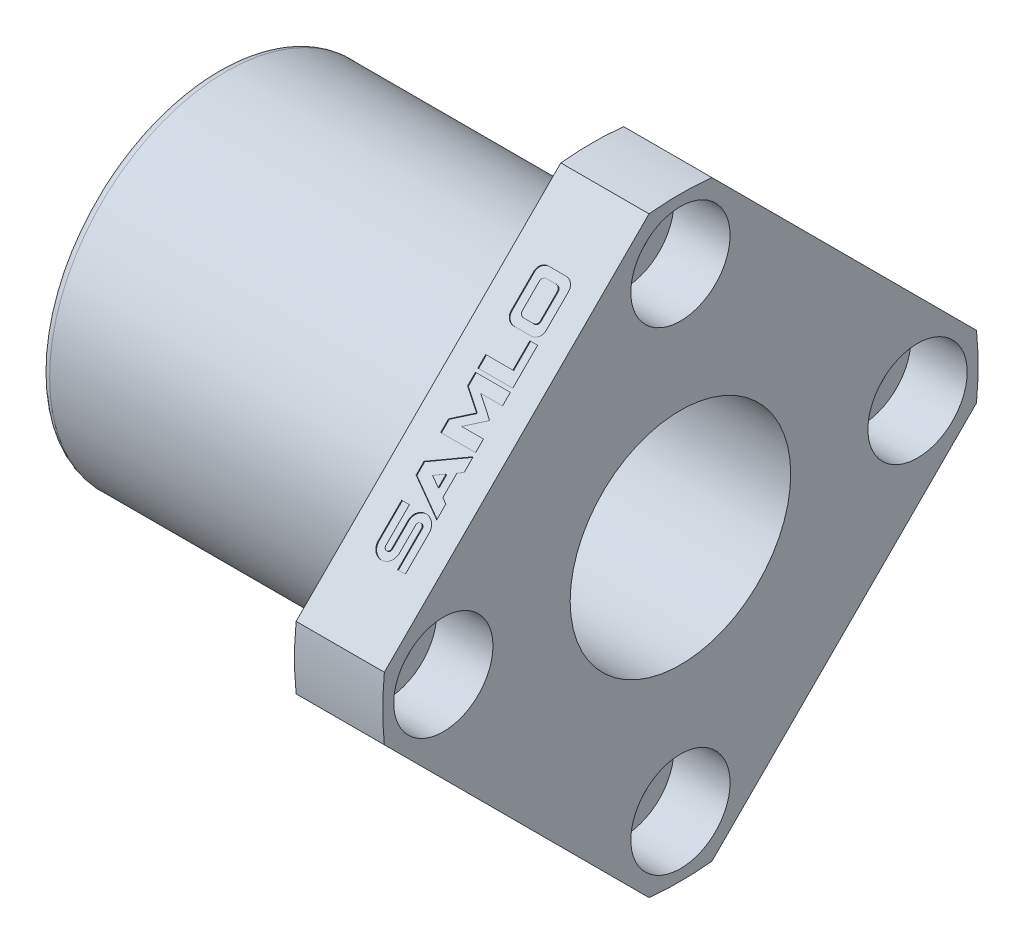
SolidWorks part; units mm, degrees
ref_plane "Front Plane" through (0, 0, 0) normal (0, 0, 1) x (1, 0, 0)
ref_plane "Top Plane" through (0, 0, 0) normal (0, 1, 0) x (1, 0, 0)
ref_plane "Right Plane" through (0, 0, 0) normal (1, 0, 0) x (0, 0, -1)
sketch "Sketch1" plane through (0, 0, 0) normal (0, 0, 1) x (1, 0, 0)
  line L0 (0, 10) -> (42, 10)
  line L1 (42, 10) -> (42, 15.2)
  line L2 (41.2, 16) -> (0.8, 16)
  line L3 (0, 15.2) -> (0, 10)
  line L4 (42, 0) -> (0, 0) construction
  arc A0 (42, 15.2) -> (41.2, 16) centre (41.2, 15.2) ccw
  arc A1 (0.8, 16) -> (0, 15.2) centre (0.8, 15.2) ccw
revolve "Revolve1" add sketch "Sketch1" angle 360 about L4
ref_plane "Plane1" through (42, 0, 0) normal (1, 0, 0) x (0, 0, -1)
sketch "Sketch2" plane through (42, 0, 0) normal (1, 0, 0) x (0, 0, -1)
  circle A0 centre (0, 0) radius 27
  circle A1 centre (21.5, 0) radius 2.75
  circle A2 centre (0, 21.5) radius 2.75
  circle A3 centre (0, -21.5) radius 2.75
  circle A4 centre (0, 0) radius 10
  circle A5 centre (-21.5, 0) radius 2.75
extrude "Boss-Extrude1" add sketch "Sketch2" against normal blind 8
sketch "Sketch3" plane through (42, 0, 0) normal (1, 0, 0) x (0, 0, -1)
  circle A0 centre (0, 21.5) radius 4.5
extrude "Cut-Extrude1" cut sketch "Sketch3" against normal blind 5.1
sketch "Sketch4" plane through (42, 0, 0) normal (1, 0, 0) x (0, 0, -1)
  line L0 (0, 21.5) -> (-21.5, 0)
  line L1 (0, 21.5) -> (21.5, 0)
pattern_linear "LPattern1" count 2 spacing 30.4056 along (0, -0.7071, 0.7071) count 2 spacing 30.4056 along (0, -0.7071, -0.7071) of "Cut-Extrude1"
sketch "Sketch5" plane through (42, 0, 0) normal (1, 0, 0) x (0, 0, -1)
  line L0 (-29.6985, 0) -> (0, -29.6985)
  line L1 (0, -29.6985) -> (29.6985, 0)
  line L2 (29.6985, 0) -> (0, 29.6985)
  line L3 (0, 29.6985) -> (-29.6985, 0)
  circle A0 centre (0, 0) radius 54
extrude "Cut-Extrude2" cut sketch "Sketch5" against normal blind 8
ref_plane "Plane2" through (0, 0, 0) normal (0, 0.7071, 0.7071) x (1, 0, 0)
ref_plane "Plane3" through (0, 14.8492, 14.8492) normal (0, 0.7071, 0.7071) x (1, 0, 0)
sketch "Sketch6" plane through (0, 14.8492, 14.8492) normal (0, 0.7071, 0.7071) x (1, 0, 0)
  line L0 (38.353, -9.8839) -> (38.353, -7.7806)
  line L1 (38.8798, -7.7806) -> (38.8798, -10.8496)
  line L2 (38.8798, -10.8496) -> (39.582, -10.8496)
  line L3 (39.582, -10.8496) -> (39.582, -7.7806)
  line L4 (37.6508, -7.7806) -> (37.6508, -9.8839)
  line L5 (37.1239, -9.8839) -> (37.1239, -6.8601)
  line L6 (37.1239, -6.8601) -> (36.4218, -6.8601)
  line L7 (36.4218, -6.8601) -> (36.4218, -9.8839)
  arc A0 (36.4218, -9.8839) -> (38.353, -9.8839) centre (37.3874, -9.869) ccw
  arc A1 (38.353, -7.7806) -> (38.8798, -7.7806) centre (38.6164, -7.7806) cw
  arc A2 (39.582, -7.7806) -> (37.6508, -7.7806) centre (38.6164, -7.7954) ccw
  arc A3 (37.6508, -9.8839) -> (37.1239, -9.8839) centre (37.3874, -9.8839) cw
extrude "Cut-Extrude3" cut sketch "Sketch6" against normal blind 0.1
sketch "Sketch7" plane through (0, 14.8492, 14.8492) normal (0, 0.7071, 0.7071) x (1, 0, 0)
  line L0 (36.4142, -5.0005) -> (39.5804, -6.8283)
  line L1 (39.5804, -6.8283) -> (39.5804, -5.6649)
  line L2 (39.5804, -5.6649) -> (39.1189, -5.3986)
  line L3 (39.1189, -5.3986) -> (39.1189, -3.5883)
  line L4 (39.1189, -3.5883) -> (39.5804, -3.3218)
  line L5 (39.5804, -3.3218) -> (39.5804, -2.1586)
  line L6 (39.5804, -2.1586) -> (36.4142, -3.9863)
  line L7 (36.4142, -3.9863) -> (36.4142, -5.0005)
  line L8 (37.5511, -4.4935) -> (38.4167, -4.9931)
  line L9 (38.4167, -4.9931) -> (38.4167, -3.9936)
  line L10 (38.4167, -3.9936) -> (37.5511, -4.4935)
extrude "Cut-Extrude4" cut sketch "Sketch7" against normal blind 0.1
sketch "Sketch8" plane through (0, 14.8492, 14.8492) normal (0, 0.7071, 0.7071) x (1, 0, 0)
  line L0 (36.4161, 2.6121) -> (36.4161, 1.6046)
  line L1 (36.4161, 1.6046) -> (38.0894, 0.3815)
  line L2 (38.0894, 0.3815) -> (36.4161, -0.8418)
  line L3 (36.4161, -0.8418) -> (36.4161, -1.8494)
  line L4 (36.4161, -1.8494) -> (39.582, -1.8494)
  line L5 (39.582, -1.8494) -> (39.582, -0.8418)
  line L6 (39.582, -0.8418) -> (37.606, -0.8418)
  line L7 (37.606, -0.8418) -> (39.2794, 0.3815)
  line L8 (39.2794, 0.3815) -> (37.606, 1.6046)
  line L9 (37.606, 1.6046) -> (39.5804, 1.6046)
  line L10 (39.5804, 1.6046) -> (39.5804, 2.6121)
  line L11 (39.5804, 2.6121) -> (36.4161, 2.6121)
extrude "Cut-Extrude5" cut sketch "Sketch8" against normal blind 0.1
sketch "Sketch9" plane through (0, 14.8492, 14.8492) normal (0, 0.7071, 0.7071) x (1, 0, 0)
  line L0 (36.4161, 2.9175) -> (39.582, 2.9175)
  line L1 (39.582, 2.9175) -> (39.582, 6.1015)
  line L2 (39.582, 6.1015) -> (38.8798, 6.1015)
  line L3 (38.8798, 6.1015) -> (38.8798, 3.925)
  line L4 (38.8798, 3.925) -> (36.4161, 3.925)
  line L5 (36.4161, 3.925) -> (36.4161, 2.9175)
extrude "Cut-Extrude6" cut sketch "Sketch9" against normal blind 0.1
sketch "Sketch10" plane through (0, 14.8492, 14.8492) normal (0, 0.7071, 0.7071) x (1, 0, 0)
  line L0 (36.4218, 10.0727) -> (36.4218, 7.1835)
  line L1 (37.1985, 6.4069) -> (38.8053, 6.4069)
  line L2 (39.582, 7.1835) -> (39.582, 10.0727)
  line L3 (38.8053, 10.8496) -> (37.1985, 10.8496)
  line L4 (37.553, 7.1701) -> (38.4506, 7.1701)
  line L5 (38.817, 7.5365) -> (38.817, 9.7198)
  line L6 (38.4506, 10.0862) -> (37.553, 10.0862)
  line L7 (37.1868, 9.7198) -> (37.1868, 7.5365)
  arc A0 (36.4218, 7.1835) -> (37.1985, 6.4069) centre (37.2007, 7.1858) ccw
  arc A1 (38.8053, 6.4069) -> (39.582, 7.1835) centre (38.803, 7.1858) ccw
  arc A2 (39.582, 10.0727) -> (38.8053, 10.8496) centre (38.803, 10.0706) ccw
  arc A3 (37.1985, 10.8496) -> (36.4218, 10.0727) centre (37.2007, 10.0706) ccw
  arc A4 (37.1868, 7.5365) -> (37.553, 7.1701) centre (37.5543, 7.5376) ccw
  arc A5 (38.4506, 7.1701) -> (38.817, 7.5365) centre (38.4494, 7.5376) ccw
  arc A6 (38.817, 9.7198) -> (38.4506, 10.0862) centre (38.4494, 9.7186) ccw
  arc A7 (37.553, 10.0862) -> (37.1868, 9.7198) centre (37.5543, 9.7186) ccw
extrude "Cut-Extrude7" cut sketch "Sketch10" against normal blind 0.1
other "Frozen***"
